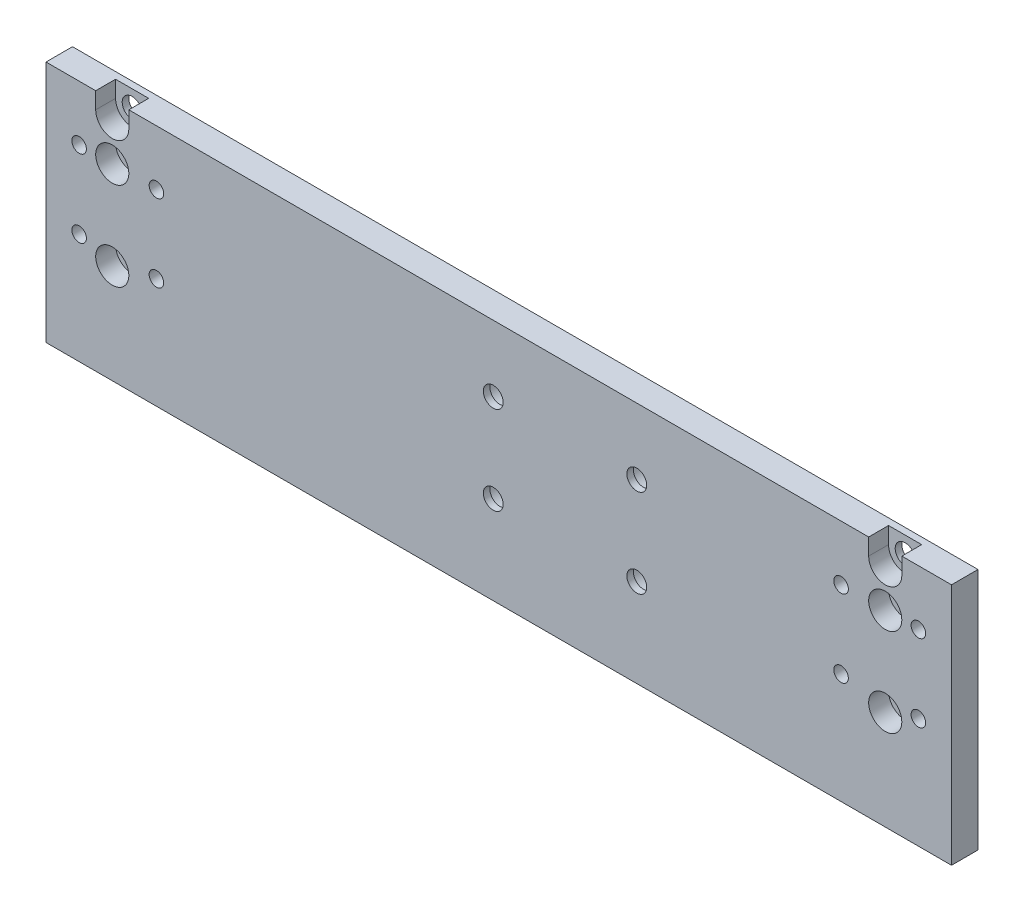
from build123d import *

# Parameters (mm, degrees)
SKETCH_1_W                 = 410
SKETCH_1_H                 = 110
EXTRUDE_1_DEPTH            = 6
HOLE_WIZARD_3_AT_2_COUNT   = 2
HOLE_WIZARD_3_AT_2_PITCH   = 35
HOLE_WIZARD_3_AT_3_COUNT   = 2
HOLE_WIZARD_3_AT_3_PITCH   = 35
HOLE_WIZARD_3_AT_4_COUNT   = 2
HOLE_WIZARD_3_AT_4_PITCH   = 49.497474683
PATTERN_LINEAR_1_COUNT     = 2
PATTERN_LINEAR_1_PITCH     = 345
HOLE_WIZARD_2_D            = 9
HOLE_WIZARD_2_DEPTH        = 12.4
HOLE_WIZARD_2_CBORE_D      = 15
HOLE_WIZARD_2_CBORE_DEPTH  = 9
HOLE_WIZARD_2_TIP          = 2.703872786
HOLE_WIZARD_3_2_AT_2_COUNT = 2
HOLE_WIZARD_3_2_AT_2_PITCH = 40
SKETCH_14_R                = 4.5
CUT_EXTRUDE_1_DEPTH        = 213.588804973
CUT_EXTRUDE_2_DEPTH        = 9
PATTERN_LINEAR_2_COUNT     = 2
PATTERN_LINEAR_2_PITCH     = 350


with BuildPart() as part:
    # 草图1 → 凸台-拉伸1 (new, symmetric)
    with BuildSketch(Plane.XY):
        Rectangle(SKETCH_1_W, SKETCH_1_H)
    extrude(amount=EXTRUDE_1_DEPTH, both=True)

    # 草图3 → Hole Wizard 3 (revolve, cut)
    with BuildSketch(Plane(origin=(190, 30, -6), x_dir=(0, 1, 0), z_dir=(1, 0, 0))):
        Polygon((0, 0), (0, 14.382840043), (3.3, 12.4), (3.3, 6.8), (5.5, 6.8), (5.5, 0), align=None)
    hole_wizard_3 = revolve(axis=Axis((190, 30, -12.35), (0, 0, 1)), mode=Mode.SUBTRACT)

    # Hole Wizard 3 at 2: Hole Wizard 3 ×2
    with Locations(*[(-i * HOLE_WIZARD_3_AT_2_PITCH, 0, 0) for i in range(1, HOLE_WIZARD_3_AT_2_COUNT)]):
        add(hole_wizard_3, mode=Mode.SUBTRACT)

    # Hole Wizard 3 at 3: Hole Wizard 3 ×2
    with Locations(*[(0, -i * HOLE_WIZARD_3_AT_3_PITCH, 0) for i in range(1, HOLE_WIZARD_3_AT_3_COUNT)]):
        add(hole_wizard_3, mode=Mode.SUBTRACT)

    # Hole Wizard 3 at 4: Hole Wizard 3 ×2
    with Locations(*[Vector(-0.7071067811865477, -0.7071067811865474, 0) * (i * HOLE_WIZARD_3_AT_4_PITCH) for i in range(1, HOLE_WIZARD_3_AT_4_COUNT)]):
        add(hole_wizard_3, mode=Mode.SUBTRACT)

    # 阵列(线性)1: Hole Wizard 3 ×2
    with Locations(*[(-i * PATTERN_LINEAR_1_PITCH, 0, 0) for i in range(1, PATTERN_LINEAR_1_COUNT)]):
        add(hole_wizard_3, mode=Mode.SUBTRACT)

    # 阵列(线性)1 copy 1 sketch → 阵列(线性)1 copy 1 (revolve, cut)
    with BuildSketch(Plane(origin=(-190, 30, -6), x_dir=(0, 1, 0), z_dir=(1, 0, 0))):
        Polygon((0, 0), (0, 14.382840043), (3.3, 12.4), (3.3, 6.8), (5.5, 6.8), (5.5, 0), align=None)
    revolve(axis=Axis((-190, 30, -12.35), (0, 0, 1)), mode=Mode.SUBTRACT)

    # 阵列(线性)1 copy 2 sketch → 阵列(线性)1 copy 2 (revolve, cut)
    with BuildSketch(Plane(origin=(-155, -5, -6), x_dir=(0, 1, 0), z_dir=(1, 0, 0))):
        Polygon((0, 0), (0, 14.382840043), (3.3, 12.4), (3.3, 6.8), (5.5, 6.8), (5.5, 0), align=None)
    revolve(axis=Axis((-155, -5, -12.35), (0, 0, 1)), mode=Mode.SUBTRACT)

    # 阵列(线性)1 copy 3 sketch → 阵列(线性)1 copy 3 (revolve, cut)
    with BuildSketch(Plane(origin=(-190, -5, -6), x_dir=(0, 1, 0), z_dir=(1, 0, 0))):
        Polygon((0, 0), (0, 14.382840043), (3.3, 12.4), (3.3, 6.8), (5.5, 6.8), (5.5, 0), align=None)
    revolve(axis=Axis((-190, -5, -12.35), (0, 0, 1)), mode=Mode.SUBTRACT)

    # 打孔尺寸(%根据)内六角圆柱头螺钉的类型2
    with Locations(Plane(origin=(62.5, 25, -6), x_dir=(-1, 0, 0), z_dir=(0, 0, -1))):
        with Locations((0, 0), (0, -40), (65, -40), (65, 0)):
            CounterBoreHole(HOLE_WIZARD_2_D / 2, HOLE_WIZARD_2_CBORE_D / 2, HOLE_WIZARD_2_CBORE_DEPTH, depth=HOLE_WIZARD_2_DEPTH)
            with Locations((0, 0, -(HOLE_WIZARD_2_DEPTH + HOLE_WIZARD_2_TIP / 2))):  # 118° drill point
                Cone(0, HOLE_WIZARD_2_D / 2, HOLE_WIZARD_2_TIP, mode=Mode.SUBTRACT)

    # 草图5 → Hole Wizard 3 2 (revolve, cut)
    with BuildSketch(Plane(origin=(-175, 30, 6), x_dir=(0, -1, 0), z_dir=(1, 0, 0))):
        Polygon((0, 0), (0, 15.103872786), (4.5, 12.4), (4.5, 9), (7.5, 9), (7.5, 0), align=None)
    hole_wizard_3_2 = revolve(axis=Axis((-175, 30, 12.35), (0, 0, -1)), mode=Mode.SUBTRACT)

    # Hole Wizard 3 2 at 2: Hole Wizard 3 2 ×2
    with Locations(*[(0, -i * HOLE_WIZARD_3_2_AT_2_PITCH, 0) for i in range(1, HOLE_WIZARD_3_2_AT_2_COUNT)]):
        add(hole_wizard_3_2, mode=Mode.SUBTRACT)

    # 草图14 → 切除-拉伸1 (cut, through all)
    with BuildSketch(Plane.XY.offset(6)):
        with Locations((-175, 47.5)):
            Circle(SKETCH_14_R)
    cut_extrude_1 = extrude(amount=-CUT_EXTRUDE_1_DEPTH, mode=Mode.SUBTRACT)

    # 草图15 → 切除-拉伸2 (cut)
    with BuildSketch(Plane.XY.offset(6)):
        with BuildLine():
            Line((-182.5, 47.5), (-182.5, 101.28932806))
            ThreePointArc((-182.5, 101.28932806), (-175, 108.78932806), (-167.5, 101.28932806))
            Line((-167.5, 101.28932806), (-167.5, 47.5))
            ThreePointArc((-167.5, 47.5), (-175, 40), (-182.5, 47.5))
        make_face()
    cut_extrude_2 = extrude(amount=-CUT_EXTRUDE_2_DEPTH, mode=Mode.SUBTRACT)

    # 阵列(线性)2: Hole Wizard 3 2, 切除-拉伸1, 切除-拉伸2 ×2
    with Locations(*[(i * PATTERN_LINEAR_2_PITCH, 0, 0) for i in range(1, PATTERN_LINEAR_2_COUNT)]):
        add(hole_wizard_3_2, mode=Mode.SUBTRACT)
        add(cut_extrude_1, mode=Mode.SUBTRACT)
        add(cut_extrude_2, mode=Mode.SUBTRACT)

    # 阵列(线性)2 copy 1 sketch → 阵列(线性)2 copy 1 (revolve, cut)
    with BuildSketch(Plane(origin=(175, -10, 6), x_dir=(0, -1, 0), z_dir=(1, 0, 0))):
        Polygon((0, 0), (0, 15.103872786), (4.5, 12.4), (4.5, 9), (7.5, 9), (7.5, 0), align=None)
    revolve(axis=Axis((175, -10, 12.35), (0, 0, -1)), mode=Mode.SUBTRACT)


solid = part.part
